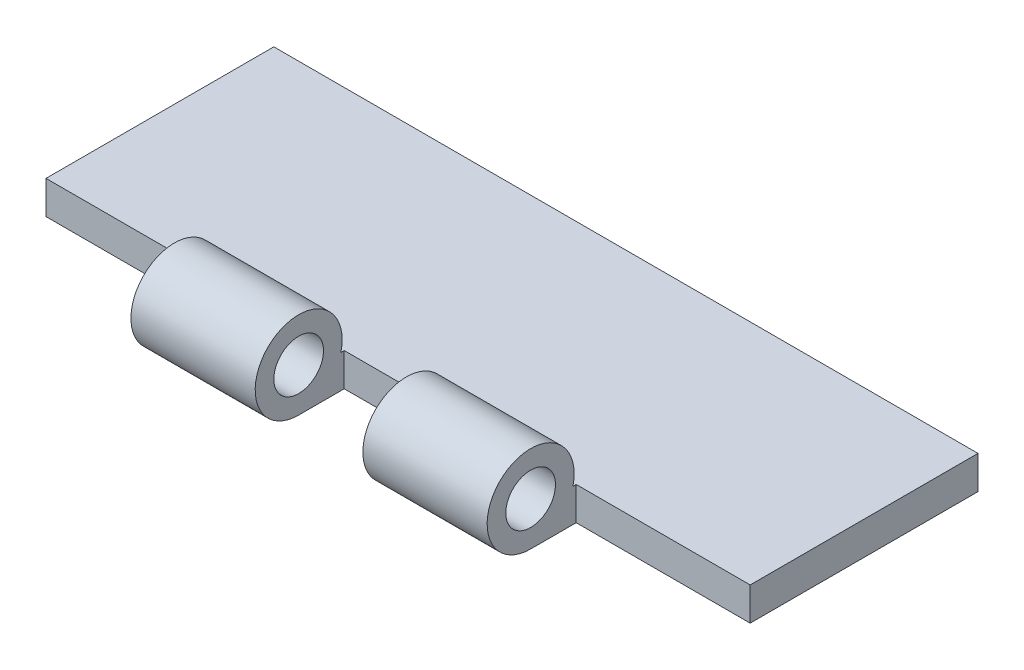
SolidWorks part; units mm, degrees
ref_plane "Front Plane" through (0, 0, 0) normal (0, 0, 1) x (1, 0, 0)
ref_plane "Top Plane" through (0, 0, 0) normal (0, 1, 0) x (1, 0, 0)
ref_plane "Right Plane" through (0, 0, 0) normal (1, 0, 0) x (0, 0, -1)
sketch "Sketch1" plane through (0, 0, 0) normal (1, 0, 0) x (0, 0, -1)
  line L0 (0, 0) -> (14.8083, 0) construction
  line L2 (33, -5.25) -> (0, -5.25)
  line L3 (33, -5.25) -> (33, -1.25)
  line L4 (33, -1.25) -> (5.099, -1.25)
  arc A0 (5.099, -1.25) -> (0, -5.25) centre (0, 0) ccw
  dimension "D1" = 10.5
  dimension "D2" = 4
  dimension "D3" = 33
extrude "Boss-Extrude1" add sketch "Sketch1" along normal mid plane 85
sketch "Sketch2" plane through (0, -1.25, 0) normal (0, 1, 0) x (1, 0, 0)
  line L0 (0, 0) -> (0, 15) construction
  line L1 (-28, 15) -> (28, 15) construction
  circle A0 centre (-28, 15) radius 3
  circle A1 centre (0, 15) radius 3
  circle A2 centre (28, 15) radius 3
  dimension "D2" = 6
  dimension "D1" = 56
  dimension "D3" = 15
extrude "Cut-Extrude1" [suppressed] cut sketch "Sketch2" against normal mid plane 10
chamfer "Chamfer1" [suppressed] distance 4 angle 45
sketch "Sketch3" plane through (0, 0, 0) normal (0, 1, 0) x (1, 0, 0)
  line L0 (0, 0) -> (42.5, 0) construction
  line L1 (21.5, 5.5) -> (21.5, -5.5) construction
  line L2 (42.5, -5.25) -> (42.5, 5.25) construction
  line L3 (0, 0) -> (0, 29.1462) construction
  line L4 (6.5, -5.5) -> (21.5, -5.5) construction
  line L5 (6.5, -5.5) -> (6.5, 5.5) construction
  line L6 (6.5, 5.5) -> (21.5, 5.5) construction
  line L8 (6.5, -5.5) -> (21.5, 5.5) construction
  line L9 (6.5, 5.5) -> (21.5, -5.5) construction
  line L10 (-6.5, 5.5) -> (-21.5, -5.5) construction
  line L11 (-6.5, -5.5) -> (-21.5, 5.5) construction
  line L12 (-21.5, -5.5) -> (-21.5, 5.5) construction
  line L13 (-6.5, 5.5) -> (-21.5, 5.5) construction
  line L14 (-6.5, -5.5) -> (-6.5, 5.5) construction
  line L15 (-6.5, -5.5) -> (-21.5, -5.5) construction
  line L29 (6.5, 5.5) -> (-6.5, 5.5)
  line L30 (6.5, 5.5) -> (6.5, -5.5)
  line L31 (6.5, -5.5) -> (-6.5, -5.5)
  line L32 (-6.5, 5.5) -> (-6.5, -5.5)
  line L33 (21.5, 5.5) -> (42.5, 5.5)
  line L34 (21.5, 5.5) -> (21.5, -5.25)
  line L35 (21.5, -5.25) -> (42.5, -5.25)
  line L36 (42.5, 5.5) -> (42.5, -5.25)
  line L37 (-21.5, 5.5) -> (-42.5, 5.5)
  line L38 (-21.5, 5.5) -> (-21.5, -5.25)
  line L39 (-21.5, -5.25) -> (-42.5, -5.25)
  line L40 (-42.5, 5.5) -> (-42.5, -5.25)
  point P7 (14, 0)
  point P15 (-14, 0)
  dimension "D1" = 15
  dimension "D2" = 11
  dimension "D3" = 6.5
extrude "Cut-Extrude2" cut sketch "Sketch3" against normal mid plane 20
sketch "Sketch4" plane through (-21.5, 0, 0) normal (-1, 0, 0) x (0, 0, 1)
  circle A0 centre (0, 0) radius 3
  dimension "D1" = 6
extrude "Cut-Extrude3" cut sketch "Sketch4" against normal through all
